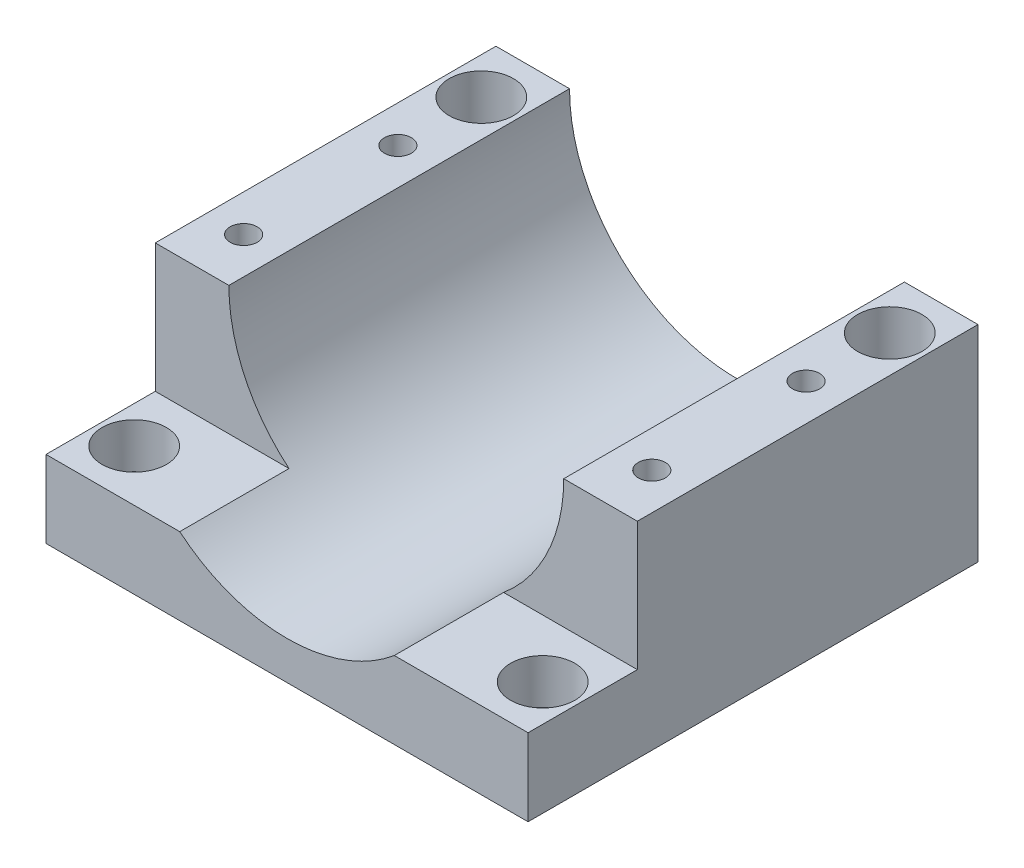
SolidWorks part; units mm, degrees
material "6061Al"
ref_plane "前视基准面" through (0, 0, 0) normal (0, 0, 1) x (1, 0, 0)
ref_plane "上视基准面" through (0, 0, 0) normal (0, 1, 0) x (1, 0, 0)
ref_plane "右视基准面" through (0, 0, 0) normal (1, 0, 0) x (0, 0, -1)
sketch "草图2" plane through (0, 0, 0) normal (0, 0, 1) x (1, 0, 0)
  line L1 (-37.5, -16) -> (37.5, -16)
  line L2 (-37.5, -16) -> (-37.5, 16)
  line L3 (-37.5, 16) -> (37.5, 16)
  line L4 (37.5, -16) -> (37.5, 16)
  line L5 (-37.5, -16) -> (37.5, 16) construction
  line L6 (-37.5, 16) -> (37.5, -16) construction
  point P0 (0, 0)
  dimension "D1" = 75
  dimension "D2" = 32
extrude "凸台-拉伸1" add sketch "草图2" along normal blind 70
sketch "草图4" plane through (0, 0, 70) normal (0, 0, 1) x (1, 0, 0)
  line L0 (37.5, 16) -> (-37.5, 16) construction
  circle A0 centre (0, 16) radius 26.05
  dimension "D1" = 52.1
extrude "切除-拉伸1" cut sketch "草图4" against normal through all
hole_wizard "M5 六角凹头螺钉的柱形沉头孔1" positions "草图5" profile "草图6" counterbore size "M5" standard "ISO" end condition through all
sketch "草图5" plane through (0, 16, 0) normal (0, 1, 0) x (1, 0, 0)
  line L0 (-31.775, 0) -> (-31.775, -70) construction
  line L1 (-26.05, 0) -> (-37.5, 0) construction
  line L2 (-26.05, -70) -> (-37.5, -70) construction
  line L4 (-37.5, -35) -> (37.5, -35) construction
  line L5 (-37.5, -70) -> (-37.5, 0) construction
  line L6 (37.5, -70) -> (37.5, 0) construction
  line L8 (0, 0) -> (0, -82.1285) construction
  line L10 (31.775, 0) -> (31.775, -70) construction
  point P0 (-31.775, -8)
  point P2 (-31.775, -62)
  point P28 (31.775, -62)
  point P29 (31.775, -8)
  dimension "D1" = 8
sketch "草图6" plane through (-31.775, 16, 8) normal (1, 0, 0) x (0, 0, 1)
  line L0 (0, 0) -> (0, 32)
  line L1 (0, 32) -> (2.75, 32)
  line L3 (2.75, 32) -> (2.75, 27)
  line L4 (2.75, 27) -> (5, 27)
  line L5 (5, 27) -> (5, 0)
  line L7 (5, 0) -> (0, 0)
  line L11 (0, -6.35) -> (0, 107.95) construction
  dimension "通孔孔直径" = 5.5
  dimension "通孔孔深度" = 32
  dimension "柱形沉头孔直径" = 10
  dimension "柱形沉头孔深度" = 27
sketch "草图7" plane through (-37.5, 0, 0) normal (-1, 0, 0) x (0, 0, 1)
  line L0 (70, 16) -> (0, 16) construction
  line L1 (53, 16) -> (70, 16)
  line L2 (53, 16) -> (53, -4)
  line L3 (53, -4) -> (70, -4)
  line L4 (70, 16) -> (70, -4)
  line L5 (70, 16) -> (70, -16) construction
  line L6 (70, -16) -> (0, -16) construction
  dimension "D1" = 17
  dimension "D2" = 12
extrude "切除-拉伸2" cut sketch "草图7" against normal through all
hole_wizard "M5 螺纹孔1" positions "草图8" profile "草图9" tap size "M5" standard "ISO"
sketch "草图8" plane through (0, 16, 0) normal (0, 1, 0) x (1, 0, 0)
  point P0 (-31.75, -21)
  point P3 (-31.75, -45)
  point P6 (31.75, -21)
  point P9 (31.75, -45)
sketch "草图9" plane through (-31.75, 16, 21) normal (1, 0, 0) x (0, 0, 1)
  line L0 (0, 0) -> (0, 13.6618)
  line L1 (0, 13.6618) -> (2.1, 12.4)
  line L2 (2.1, 12.4) -> (2.1, 0)
  line L5 (2.1, 0) -> (0, 0)
  line L10 (0, 13.6618) -> (-2.1, 12.4) construction
  line L11 (0, -6.35) -> (0, 107.95) construction
  dimension "螺纹孔钻头直径" = 4.2
  dimension "螺纹孔钻头深度" = 12.4
  dimension "导头角度" = 118
cosmetic thread "孔螺蚊线1" parameters "D1"=10, "D2"=5
cosmetic thread "孔螺蚊线2" parameters "D1"=10, "D2"=5
cosmetic thread "孔螺蚊线3" parameters "D1"=10, "D2"=5
cosmetic thread "孔螺蚊线4" parameters "D1"=10, "D2"=5
